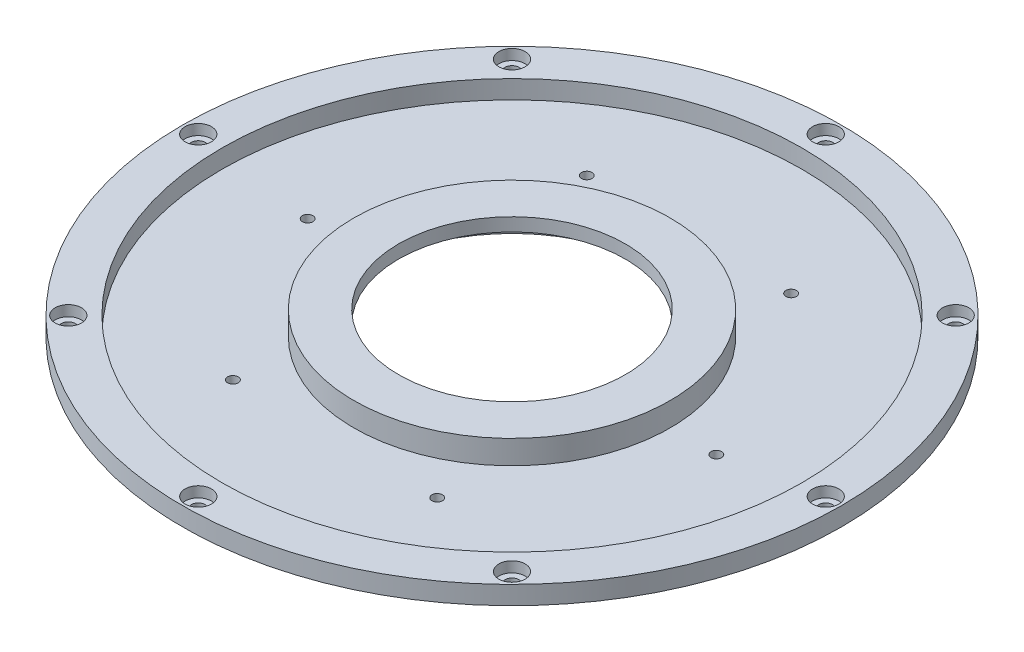
SolidWorks part; units mm, degrees
material "1060 合金"
ref_plane "Front Plane" through (0, 0, 0) normal (0, 0, 1) x (1, 0, 0)
ref_plane "Top Plane" through (0, 0, 0) normal (0, 1, 0) x (1, 0, 0)
ref_plane "Right Plane" through (0, 0, 0) normal (1, 0, 0) x (0, 0, -1)
sketch "Sketch1" plane through (0, 0, 0) normal (0, 0, 1) x (1, 0, 0)
  line L0 (0, 0) -> (0, -18.4841) construction
  line L1 (-125, 132) -> (-115, 132)
  line L2 (-115, 132) -> (-115, 127)
  line L3 (-115, 127) -> (-55, 127)
  line L5 (-55, 127) -> (-55, 136)
  line L6 (-55, 136) -> (-43, 136)
  line L7 (-43, 136) -> (-43, 141)
  line L8 (-43, 141) -> (-60, 141)
  line L9 (-60, 141) -> (-60, 132)
  line L10 (115, 132) -> (-115, 132) construction
  line L11 (-60, 132) -> (-110, 132)
  line L12 (-110, 132) -> (-110, 139)
  line L13 (-110, 139) -> (-125, 139)
  line L14 (-125, 139) -> (-125, 132)
revolve "Revolve1" add sketch "Sketch1" angle 360 about L0
sketch "Sketch2" plane through (0, 139, 0) normal (0, 1, 0) x (1, 0, 0)
  circle A0 centre (0, 119) radius 2.65
  circle A2 centre (0, 0) radius 110 construction
  circle A3 centre (84.1457, 84.1457) radius 2.65
  circle A4 centre (119, 0) radius 2.65
  circle A5 centre (84.1457, -84.1457) radius 2.65
  circle A6 centre (0, -119) radius 2.65
  circle A7 centre (-84.1457, -84.1457) radius 2.65
  circle A8 centre (-119, 0) radius 2.65
  circle A9 centre (-84.1457, 84.1457) radius 2.65
  point P21 (0, 0)
  dimension "D1" = 119
extrude "Cut-Extrude1" cut sketch "Sketch2" against normal blind 10
sketch "Sketch3" plane through (0, 139, 0) normal (0, 1, 0) x (1, 0, 0)
  circle A0 centre (0, 119) radius 5
  circle A1 centre (84.1457, 84.1457) radius 5
  circle A2 centre (119, 0) radius 5
  circle A3 centre (84.1457, -84.1457) radius 5
  circle A4 centre (0, -119) radius 5
  circle A5 centre (-84.1457, -84.1457) radius 5
  circle A6 centre (-119, 0) radius 5
  circle A7 centre (-84.1457, 84.1457) radius 5
  point P20 (0, 0)
  dimension "D1" = 8
extrude "Cut-Extrude3" cut sketch "Sketch3" against normal blind 4 contours A0
sketch "Sketch4" plane through (0, 132, 0) normal (0, 1, 0) x (1, 0, 0)
  circle A0 centre (77.5, 0) radius 2
  circle A1 centre (38.75, -67.117) radius 2
  circle A2 centre (-38.75, -67.117) radius 2
  circle A3 centre (-77.5, 0) radius 2
  circle A4 centre (-38.75, 67.117) radius 2
  circle A5 centre (38.75, 67.117) radius 2
  point P15 (0, 0)
  dimension "D1" = 6
extrude "Cut-Extrude4" cut sketch "Sketch4" against normal blind 20
